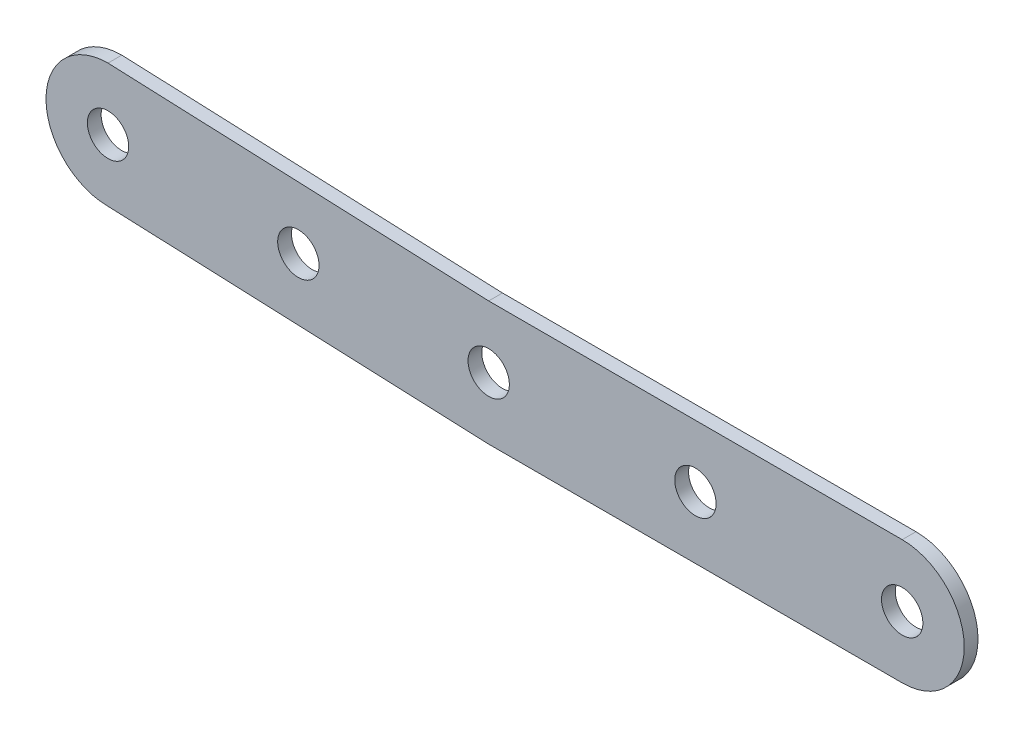
from build123d import *

# Parameters (mm, degrees)
SKETCH1_R           = 3
BOSS_EXTRUDE1_DEPTH = 2


with BuildPart() as part:
    # Sketch1 → Boss-Extrude1 (new body)
    with BuildSketch(Plane.XY):
        with BuildLine():
            Line((0, 9), (55.234065112, 6.728534899))
            Line((55.234065112, 6.728534899), (115.234079808, 6.728534899))
            ThreePointArc((115.234079808, 6.728534899), (124.234079808, -2.271465101), (115.234079808, -11.271465101))
            Line((115.234079808, -11.271465101), (55.234065112, -11.271465101))
            Line((55.234065112, -11.271465101), (0, -9))
            ThreePointArc((0, -9), (-9, 0), (0, 9))
        make_face()
        Circle(SKETCH1_R, mode=Mode.SUBTRACT)
        with Locations((55.234065112, -2.271465101)):
            Circle(SKETCH1_R, mode=Mode.SUBTRACT)
        with Locations((115.234079808, -2.271465101)):
            Circle(SKETCH1_R, mode=Mode.SUBTRACT)
        with Locations((27.617032556, -1.13573255)):
            Circle(SKETCH1_R, mode=Mode.SUBTRACT)
        with Locations((85.23407246, -2.271465101)):
            Circle(SKETCH1_R, mode=Mode.SUBTRACT)
    extrude(amount=BOSS_EXTRUDE1_DEPTH)


solid = part.part
